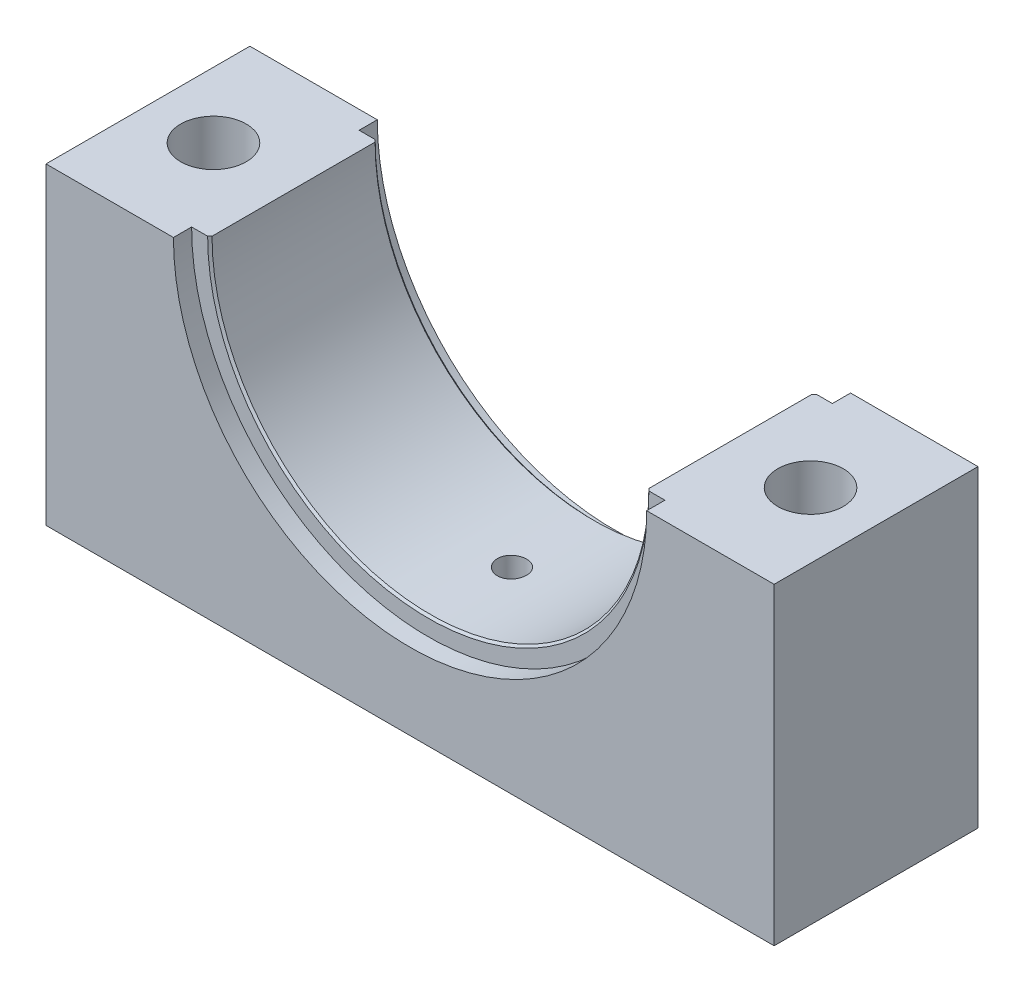
from build123d import *

# Parameters (mm, degrees)
BOSS_EXTRUDE1_DEPTH = 28
SKETCH2_R           = 32.5
CUT_EXTRUDE1_DEPTH  = 2.5
CUT_EXTRUDE2_START  = -2.5
SKETCH3_R           = 32.5
CUT_EXTRUDE2_DEPTH  = 2.5
CHAMFER1_SIZE       = 0.3
HOLE1_D             = 9
HOLE2_D             = 4
HOLE2_DEPTH         = 34


with BuildPart() as part:
    # Sketch1 → Boss-Extrude1 (new body)
    with BuildSketch(Plane.XY):
        with BuildLine():
            Line((-50, 0), (-30, 0))
            ThreePointArc((-30, 0), (0, -30), (30, 0))
            Line((30, 0), (50, 0))
            Line((50, 0), (50, -43))
            Line((50, -43), (-50, -43))
            Line((-50, -43), (-50, 0))
        make_face()
    extrude(amount=BOSS_EXTRUDE1_DEPTH)

    # Sketch2 → Cut-Extrude1 (cut)
    with BuildSketch(Plane.XY.offset(28)):
        Circle(SKETCH2_R)
    extrude(amount=-CUT_EXTRUDE1_DEPTH, mode=Mode.SUBTRACT)

    # Sketch3 → Cut-Extrude2 (cut)
    with BuildSketch(Plane(origin=(0, 0, 0), x_dir=(-1, 0, 0), z_dir=(0, 0, -1)).offset(CUT_EXTRUDE2_START)):
        Circle(SKETCH3_R)
    extrude(amount=CUT_EXTRUDE2_DEPTH, mode=Mode.SUBTRACT)

    # Chamfer1
    chamfer1_edges = [part.edges().sort_by_distance(p)[0] for p in [
        (0, -30, 25.5),
        (0, -30, 2.5),
    ]]
    chamfer(chamfer1_edges, length=CHAMFER1_SIZE)

    # Hole1 (through all)
    with Locations(Plane(origin=(0, 0, 0), x_dir=(1, 0, 0), z_dir=(0, 1, 0))):
        with Locations((-41, -14), (41, -14)):
            Hole(HOLE1_D / 2)

    # Hole2
    with Locations(Plane(origin=(0, 0, 0), x_dir=(1, 0, 0), z_dir=(0, 1, 0))):
        with Locations((0, -14)):
            Hole(HOLE2_D / 2, depth=HOLE2_DEPTH)


solid = part.part
